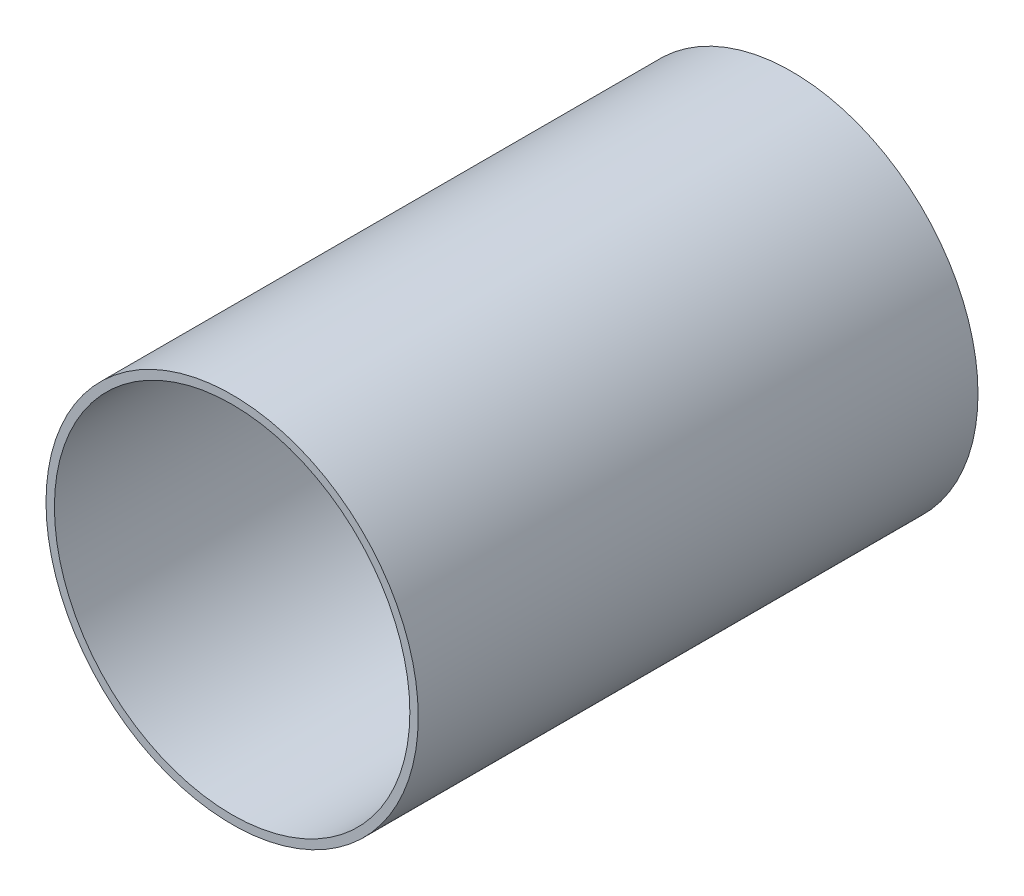
SolidWorks part; units mm, degrees
material "AISI 304"
ref_plane "Front Plane" through (0, 0, 0) normal (0, 0, 1) x (1, 0, 0)
ref_plane "Top Plane" through (0, 0, 0) normal (0, 1, 0) x (1, 0, 0)
ref_plane "Right Plane" through (0, 0, 0) normal (1, 0, 0) x (0, 0, -1)
sketch "Sketch1" plane through (0, 0, 0) normal (0, 0, 1) x (1, 0, 0)
  circle A0 centre (0, 0) radius 66.5
  circle A1 centre (0, 0) radius 63.5
  dimension "D1" = 133
  dimension "D2" = 3
extrude "Boss-Extrude1" add sketch "Sketch1" along normal blind 200
